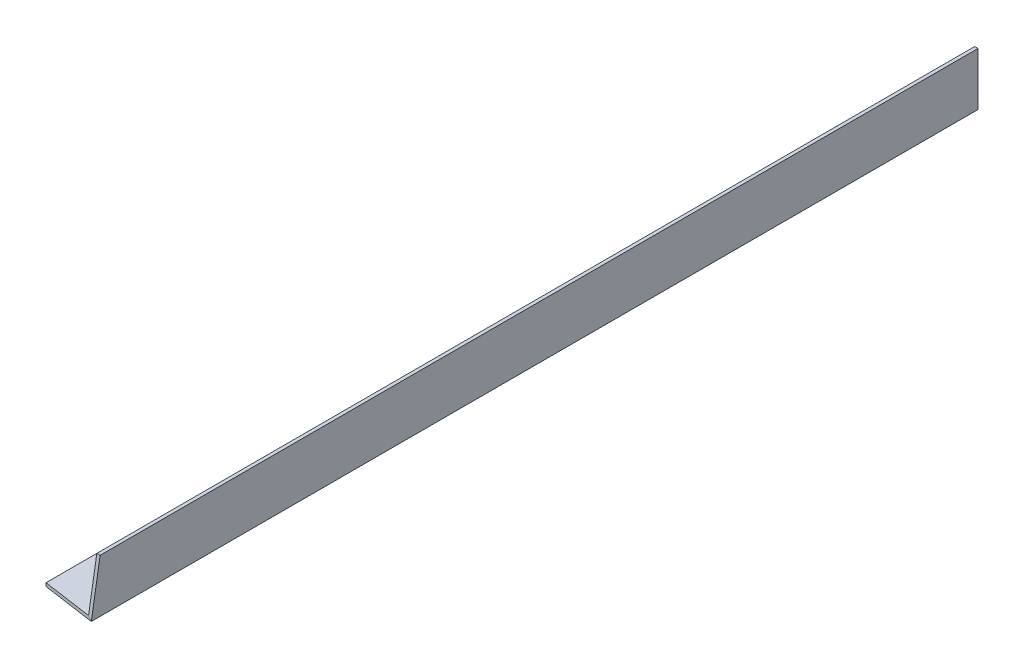
SolidWorks part; units mm, degrees
material "AISI 1045 钢，冷拔"
ref_plane "Front Plane" through (0, 0, 0) normal (0, 0, 1) x (1, 0, 0)
ref_plane "Top Plane" through (0, 0, 0) normal (0, 1, 0) x (1, 0, 0)
ref_plane "Right Plane" through (0, 0, 0) normal (1, 0, 0) x (0, 0, -1)
sketch "Sketch1" plane through (0, 0, 0) normal (0, 0, 1) x (1, 0, 0)
  line L0 (-127, 0) -> (0, 0)
  line L1 (55, 0) -> (-55, 0) construction
  line L2 (0, 0) -> (0, 127)
  line L3 (0, -55) -> (0, 55) construction
  line L4 (0, 127) -> (-7.9375, 127)
  line L5 (-7.9375, 127) -> (-7.9375, 7.9375)
  line L6 (-7.9375, 7.9375) -> (-127, 7.9375)
  line L7 (-127, 7.9375) -> (-127, 0)
  dimension "D1" = 7.9375
  dimension "D2" = 127
extrude "Boss-Extrude1" add sketch "Sketch1" along normal mid plane 2127.631
sketch "Sketch2" plane through (0, 0, 0) normal (1, 0, 0) x (0, 0, -1)
  line L0 (-1063.8155, 0) -> (-1063.8155, 127)
  line L1 (69.85, 0) -> (-69.85, 0) construction
  line L2 (-1063.8155, 0) -> (-1063.8155, 127) construction
  line L3 (-1063.8155, 127) -> (-1042.6769, 127)
  line L4 (-1063.8155, 127) -> (1063.8155, 127) construction
  line L5 (-1042.6769, 127) -> (-1063.8155, 0)
  dimension "D1" = 9.45
extrude "Cut-Extrude1" cut sketch "Sketch2" against normal blind 150
sketch "Sketch3" plane through (0, 0, 0) normal (0, -1, 0) x (1, 0, 0)
  line L0 (0, 1063.8155) -> (-127, 1063.8155)
  line L1 (-127, 1063.8155) -> (-127, 1045.5598)
  line L2 (-127, 1063.8155) -> (-127, -1063.8155) construction
  line L3 (-127, 1045.5598) -> (0, 1063.8155)
  line L4 (-63.5, -880.4592) -> (-63.5, -916.9717) construction
  line L5 (-56.3563, -880.4592) -> (-56.3562, -916.9717)
  line L6 (-70.6438, -880.4592) -> (-70.6437, -916.9717)
  line L7 (-127, -1063.8155) -> (0, -1063.8155) construction
  arc A0 (-56.3563, -880.4592) -> (-70.6438, -880.4592) centre (-63.5, -880.4592) ccw
  arc A1 (-70.6437, -916.9717) -> (-56.3562, -916.9717) centre (-63.5, -916.9717) ccw
  circle A2 centre (-88.9, 879.2845) radius 7.1437
  point P9 (-63.5, -898.7155)
  dimension "D2" = 7.1437
  dimension "D6" = 14.2875
  dimension "D1" = 8.18
  dimension "D3" = 36.5125
  dimension "D4" = 165.1
  dimension "D5" = 63.5
  dimension "D7" = 38.1
  dimension "D8" = 1778
extrude "Cut-Extrude2" cut sketch "Sketch3" against normal blind 150
